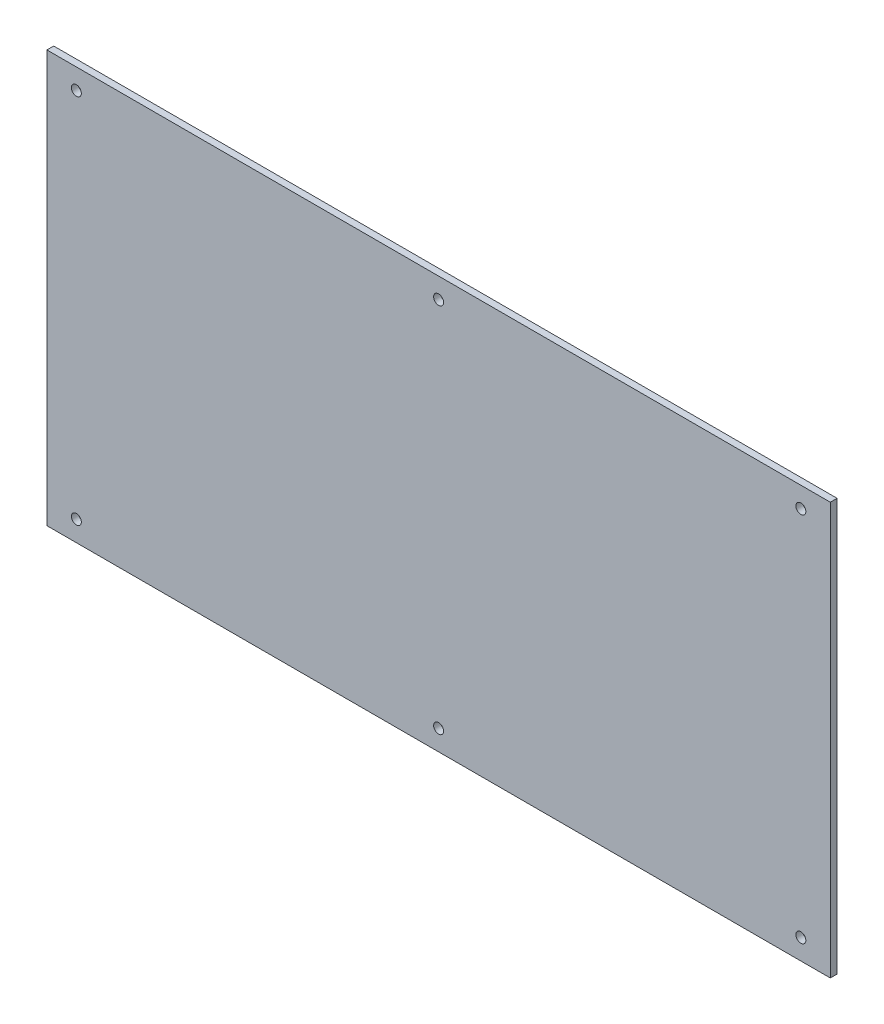
from build123d import *

# Parameters (mm, degrees)
SKETCH_1_W          = 346
SKETCH_1_H          = 182
EXTRUDE_1_DEPTH     = 3
SKETCH_2_R          = 2.2
CUT_EXTRUDE_1_DEPTH = 10


with BuildPart() as part:
    # 草图1 → 凸台-拉伸1 (new body)
    with BuildSketch(Plane.XY):
        Rectangle(SKETCH_1_W, SKETCH_1_H)
    extrude(amount=EXTRUDE_1_DEPTH)

    # 草图2 → 切除-拉伸1 (cut)
    with BuildSketch(Plane(origin=(0, 0, 0), x_dir=(-1, 0, 0), z_dir=(0, 0, -1))):
        with Locations((0, 82)):
            Circle(SKETCH_2_R)
        with Locations((160, 82)):
            Circle(SKETCH_2_R)
        with Locations((0, -82)):
            Circle(SKETCH_2_R)
        with Locations((160, -82)):
            Circle(SKETCH_2_R)
        with Locations((-160, -82)):
            Circle(SKETCH_2_R)
        with Locations((-160, 82)):
            Circle(SKETCH_2_R)
    extrude(amount=-CUT_EXTRUDE_1_DEPTH, mode=Mode.SUBTRACT)


solid = part.part
